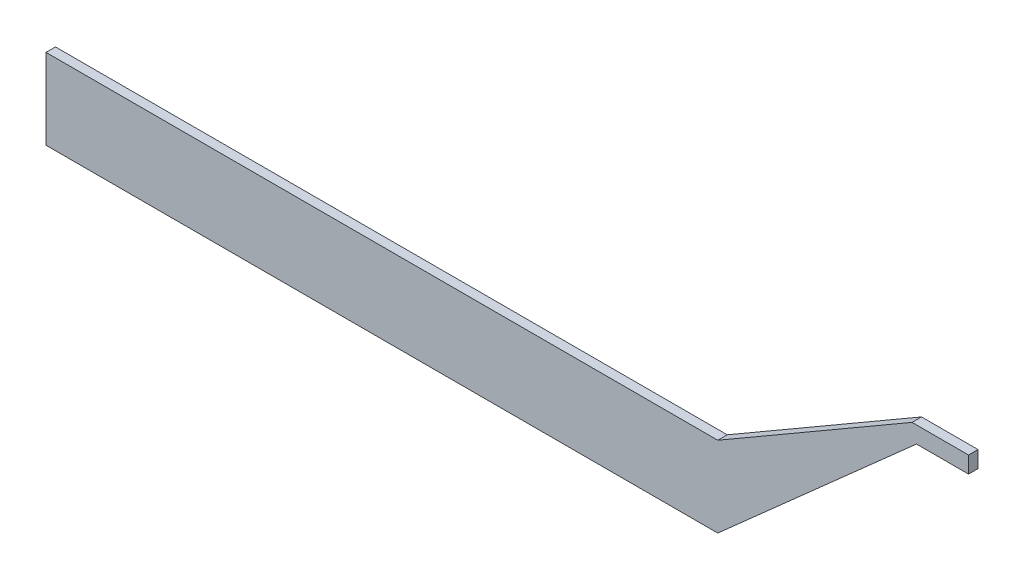
SolidWorks part; units mm, degrees
ref_plane "Front Plane" through (0, 0, 0) normal (0, 0, 1) x (1, 0, 0)
ref_plane "Top Plane" through (0, 0, 0) normal (0, 1, 0) x (1, 0, 0)
ref_plane "Right Plane" through (0, 0, 0) normal (1, 0, 0) x (0, 0, -1)
sketch "Sketch1" plane through (0, 0, 0) normal (0, 0, 1) x (1, 0, 0)
  line L0 (14.2, 1.7) -> (18.3057, 4.08)
  line L1 (0, 0) -> (14.1988, 0)
  line L2 (0, 0) -> (0, 1.7)
  line L3 (18.3057, 4.08) -> (19.5, 4.08)
  line L4 (19.5, 3.73) -> (19.5, 4.08)
  line L5 (19.5, 3.73) -> (18.4, 3.73)
  line L6 (18.4, 3.73) -> (14.1988, 0)
  line L7 (0, 1.7) -> (14.2, 1.7)
  dimension "D1" = 19.5
  dimension "D2" = 0.35
  dimension "D3" = 1.7
  dimension "D4" = 2.03
  dimension "D5" = 5.3
  dimension "D6" = 41.6
  dimension "D7" = 30.1
  dimension "D8" = 1.1
extrude "Boss-Extrude1" add sketch "Sketch1" along normal blind 0.2
